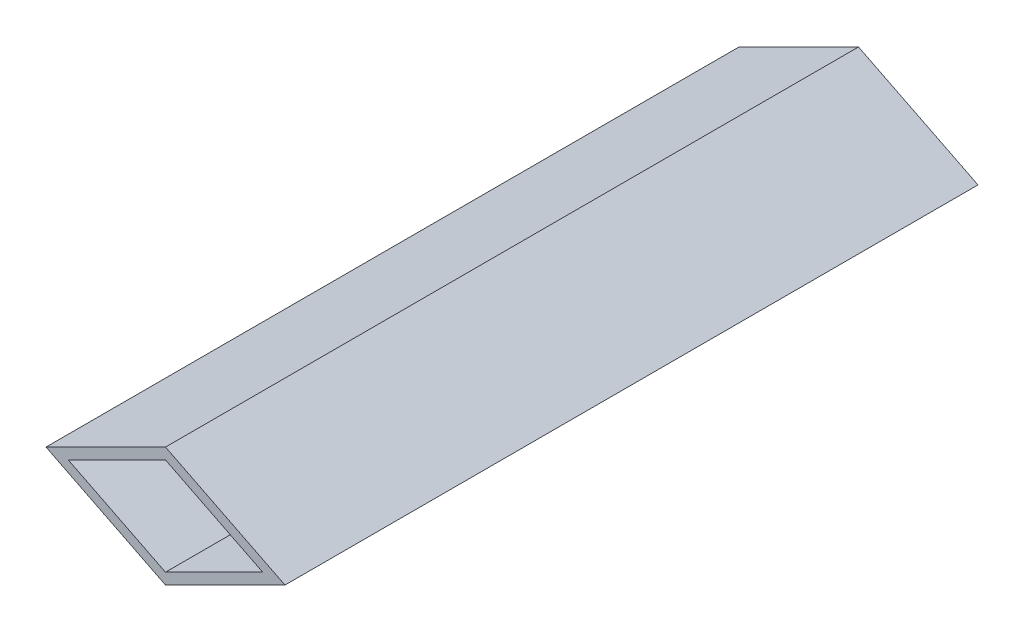
from build123d import *

# Parameters (mm, degrees)
BOSS_EXTRUDE1_DEPTH = 348
CUT_EXTRUDE1_DEPTH  = 350


with BuildPart() as part:
    # Sketch1 → Boss-Extrude1 (new body)
    with BuildSketch(Plane.XY):
        Polygon((0, 169.911519959), (-60, 139.911519959), (0, 109.911519959), (60, 139.911519959), align=None)
    extrude(amount=BOSS_EXTRUDE1_DEPTH)

    # Sketch2 → Cut-Extrude1 (cut)
    with BuildSketch(Plane.XY.offset(348)):
        Polygon((48.819660113, 139.911519959), (0, 164.321350015), (-48.819660113, 139.911519959), (0, 115.501689902), align=None)
    extrude(amount=-CUT_EXTRUDE1_DEPTH, mode=Mode.SUBTRACT)


solid = part.part
